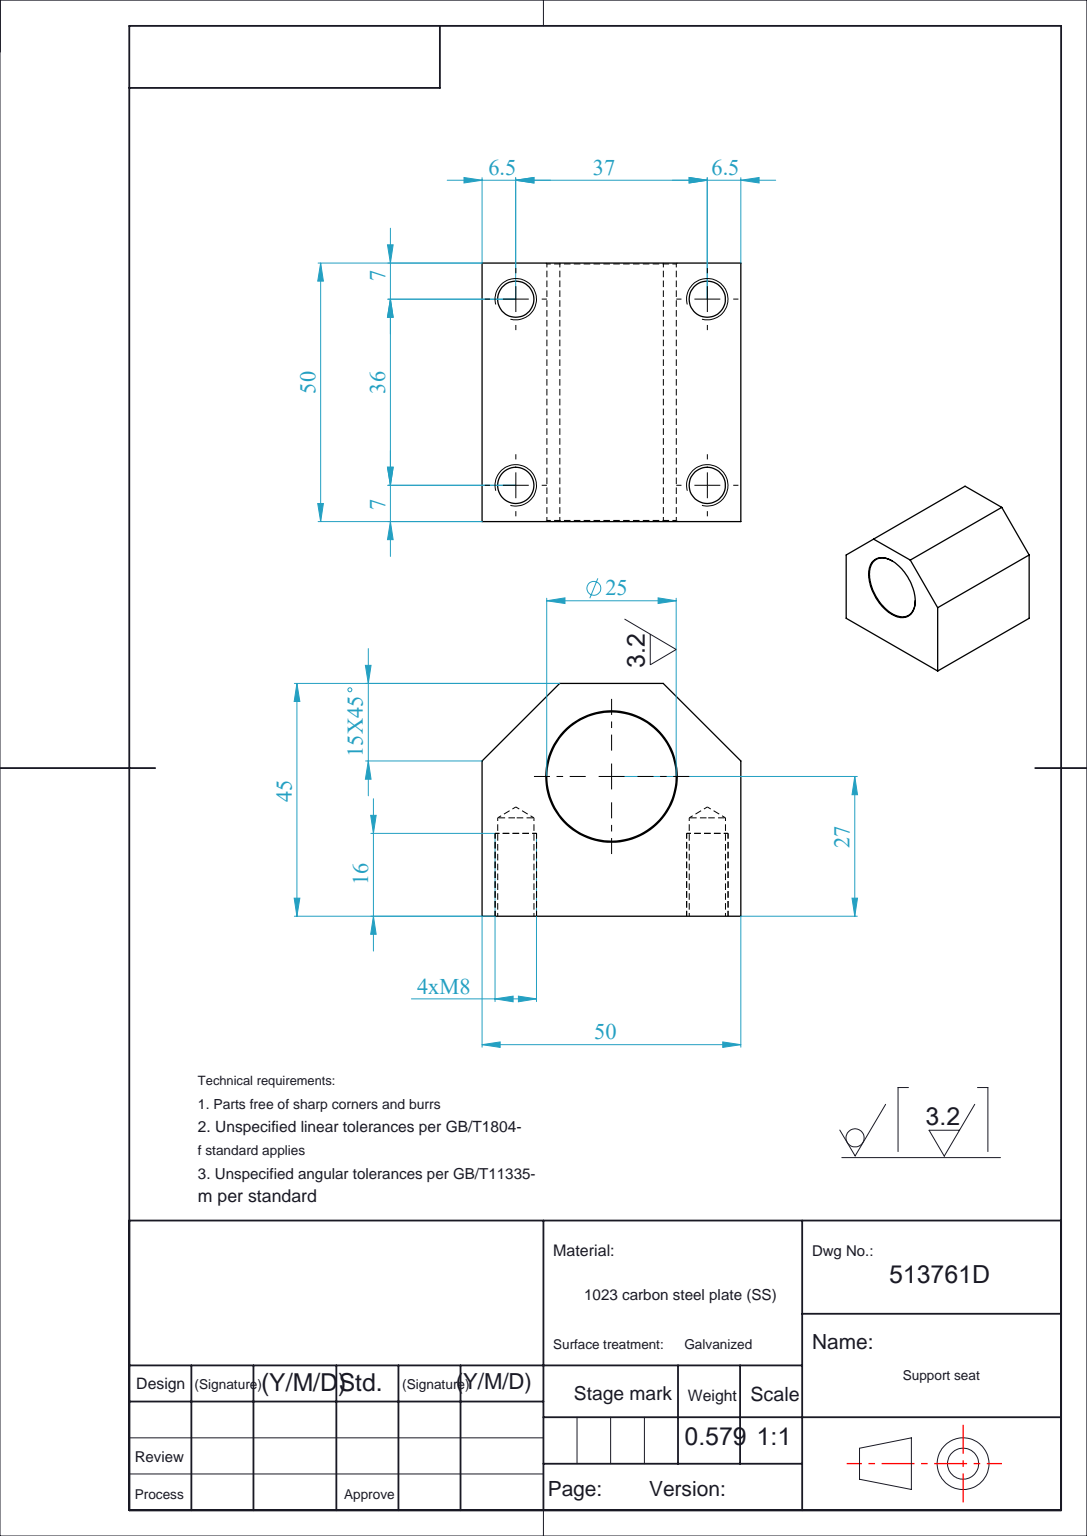
from build123d import *

# Parameters (mm, degrees)
SKETCH1_W                 = 50
SKETCH1_H                 = 50
BOSS_EXTRUDE1_DEPTH       = 45
SKETCH3_R                 = 12.5
CUT_EXTRUDE1_DEPTH        = 56
CHAMFER1_SIZE             = 15
M8X1_0_TAPPED_HOLE1_D     = 7
M8X1_0_TAPPED_HOLE1_DEPTH = 19
M8X1_0_TAPPED_HOLE1_TIP   = 2.103012167
CHAMFER2_SIZE             = 0.2
CHAMFER3_SIZE             = 0.2


with BuildPart() as part:
    # Sketch1 → Boss-Extrude1 (new body)
    with BuildSketch(Plane.XY):
        Rectangle(SKETCH1_W, SKETCH1_H)
    extrude(amount=BOSS_EXTRUDE1_DEPTH)

    # Sketch3 → Cut-Extrude1 (cut)
    with BuildSketch(Plane(origin=(25, 0, 0), x_dir=(0, 0, -1), z_dir=(1, 0, 0))):
        with Locations(Location((-27, 0, 0), (0, 0, 90))):
            Circle(SKETCH3_R)
    extrude(amount=-CUT_EXTRUDE1_DEPTH, mode=Mode.SUBTRACT)

    # Chamfer1
    chamfer1_edges = [part.edges().sort_by_distance(p)[0] for p in [
        (0, -25, 45),
        (0, 25, 45),
    ]]
    chamfer(chamfer1_edges, length=CHAMFER1_SIZE)

    # M8x1.0 Tapped Hole1
    with Locations(Plane(origin=(0, 0, 0), x_dir=(-1, 0, 0), z_dir=(0, 0, -1))):
        with Locations((-18, 18.5), (18, 18.5), (18, -18.5), (-18, -18.5)):
            Hole(M8X1_0_TAPPED_HOLE1_D / 2, depth=M8X1_0_TAPPED_HOLE1_DEPTH)
            with Locations((0, 0, -(M8X1_0_TAPPED_HOLE1_DEPTH + M8X1_0_TAPPED_HOLE1_TIP / 2))):  # 118° drill point
                Cone(0, M8X1_0_TAPPED_HOLE1_D / 2, M8X1_0_TAPPED_HOLE1_TIP, mode=Mode.SUBTRACT)

    # Chamfer2
    chamfer2_edges = [part.edges().sort_by_distance(p)[0] for p in [
        (25, -12.5, 27),
    ]]
    chamfer(chamfer2_edges, length=CHAMFER2_SIZE)

    # Chamfer3
    chamfer3_edges = [part.edges().sort_by_distance(p)[0] for p in [
        (-25, -12.5, 27),
    ]]
    chamfer(chamfer3_edges, length=CHAMFER3_SIZE)


solid = part.part
